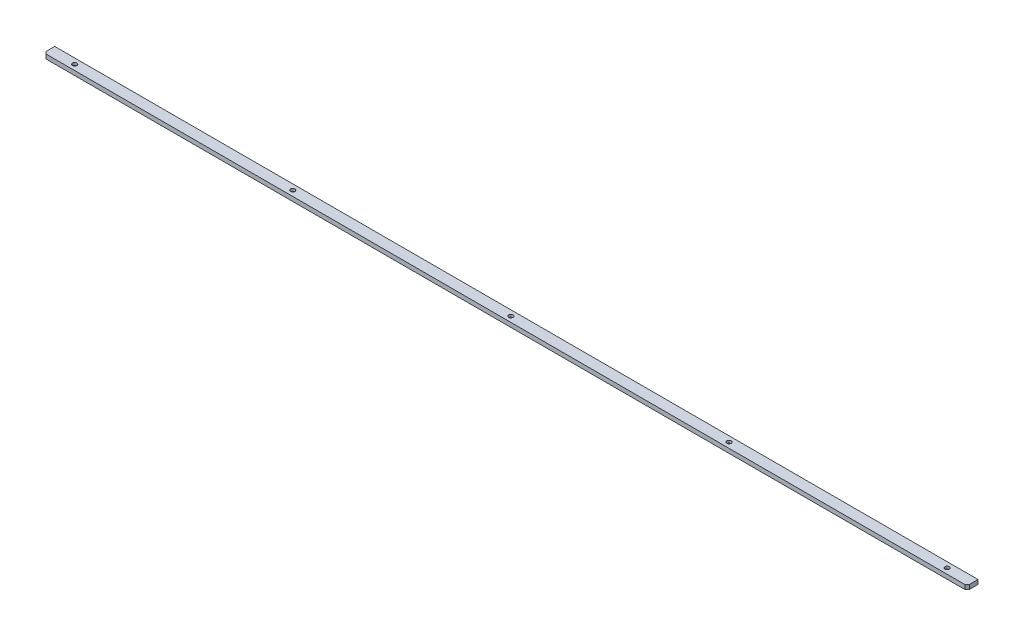
SolidWorks part; units mm, degrees
material "黑色POM "
ref_plane "前基準面" through (0, 0, 0) normal (0, 0, 1) x (1, 0, 0)
ref_plane "上基準面" through (0, 0, 0) normal (0, 1, 0) x (1, 0, 0)
ref_plane "右基準面" through (0, 0, 0) normal (1, 0, 0) x (0, 0, -1)
sketch "草图1" plane through (0, 0, 0) normal (0, 1, 0) x (1, 0, 0)
  line L1 (-635, -7.5) -> (635, -7.5)
  line L2 (-635, -7.5) -> (-635, 7.5)
  line L3 (-635, 7.5) -> (635, 7.5)
  line L4 (635, -7.5) -> (635, 7.5)
  line L5 (-635, -7.5) -> (635, 7.5) construction
  line L6 (-635, 7.5) -> (635, -7.5) construction
  point P0 (0, 0)
  dimension "D1" = 1270
  dimension "D2" = 15
extrude "凸台-拉伸1" add sketch "草图1" along normal mid plane 6
chamfer "倒角1" distance 3 angle 45 2 edges at (-635, 0, 7.5) (635, 0, 7.5)
hole_wizard "打孔尺寸(%根据)内六角圆柱头螺钉的类型1" positions "草图2" profile "草图3" counterbore size "M3" standard "GB" end condition through all
sketch "草图2" plane through (0, 3, 0) normal (0, 1, 0) x (1, 0, 0)
  point P0 (-600, 0)
  point P5 (-300, 0)
  point P6 (0, 0)
  point P7 (300, 0)
  point P8 (600, 0)
  dimension "D2" = 300
  dimension "D1" = 5
sketch "草图3" plane through (-600, 3, 0) normal (1, 0, 0) x (0, 0, 1)
  line L0 (0, 0) -> (0, 6)
  line L1 (0, 6) -> (1.7, 6)
  line L3 (1.7, 6) -> (1.7, 3.4)
  line L4 (1.7, 3.4) -> (3, 3.4)
  line L5 (3, 3.4) -> (3, 0)
  line L7 (3, 0) -> (0, 0)
  line L11 (0, -6.35) -> (0, 107.95) construction
  dimension "通孔孔直径" = 3.4
  dimension "通孔孔深度" = 6
  dimension "柱形沉头孔直径" = 6
  dimension "柱形沉头孔深度" = 3.4
